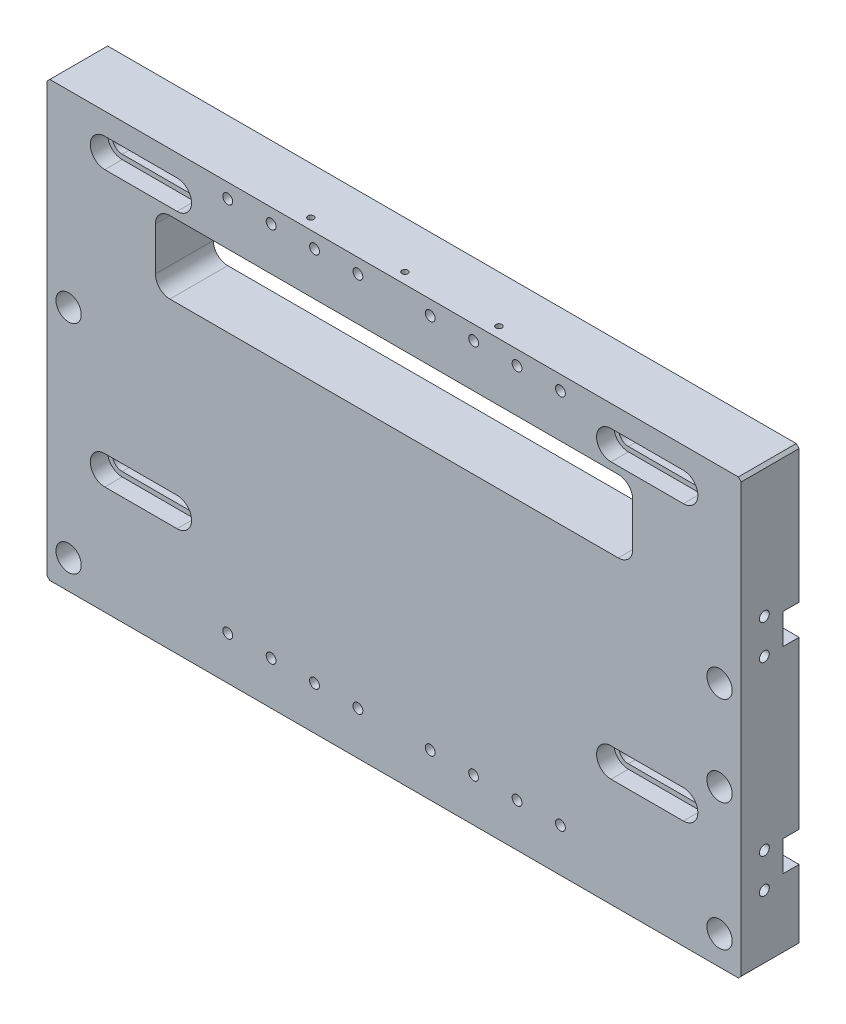
from build123d import *

# Parameters (mm, degrees)
SKETCH1_W                                            = 480
SKETCH1_H                                            = 300
BOSS_EXTRUDE1_DEPTH                                  = 20
CUT_EXTRUDE1_DEPTH                                   = 286.832118559
HOLE_SIZE_PER_SOCKET_HEAD_CAP_SCREW_TYPE_D           = 17.5
HOLE_SIZE_PER_SOCKET_HEAD_CAP_SCREW_TYPE_CBORE_D     = 26
HOLE_SIZE_PER_SOCKET_HEAD_CAP_SCREW_TYPE_CBORE_DEPTH = 17.5
CBORE_FOR_M12_HEX_SOCKET_HEAD_CAP_SCREW1_D           = 13.5
CBORE_FOR_M12_HEX_SOCKET_HEAD_CAP_SCREW1_CBORE_D     = 20
CBORE_FOR_M12_HEX_SOCKET_HEAD_CAP_SCREW1_CBORE_DEPTH = 12
SKETCH7_W                                            = 11
SKETCH7_H                                            = 21
CUT_EXTRUDE2_DEPTH                                   = 504.289181286
M5_TAPPED_HOLE1_D                                    = 4.2
M5_TAPPED_HOLE1_DEPTH                                = 12.4
M5_TAPPED_HOLE1_TIP                                  = 1.2618073
CUT_EXTRUDE5_START                                   = -100
CUT_EXTRUDE5_DEPTH                                   = 100
CUT_EXTRUDE6_DEPTH                                   = 12
CHAMFER1_SIZE                                        = 2
M8_TAPPED_HOLE1_D                                    = 6.8
M8_TAPPED_HOLE1_DEPTH                                = 19.75
M8_TAPPED_HOLE1_TIP                                  = 2.042926105
SKETCH29_R                                           = 11
CUT_EXTRUDE7_DEPTH                                   = 130
SKETCH30_R                                           = 14.25
CUT_EXTRUDE8_DEPTH                                   = 30
M6_TAPPED_HOLE2_D                                    = 5
M6_TAPPED_HOLE2_DEPTH                                = 15
M6_TAPPED_HOLE2_TIP                                  = 1.502151548
M8_TAPPED_HOLE2_AT_2_COUNT                           = 2
M8_TAPPED_HOLE2_AT_2_PITCH                           = 24
M8_TAPPED_HOLE2_AT_3_COUNT                           = 2
M8_TAPPED_HOLE2_AT_3_PITCH                           = 116
M8_TAPPED_HOLE2_AT_4_COUNT                           = 2
M8_TAPPED_HOLE2_AT_4_PITCH                           = 140


with BuildPart() as part:
    # Sketch1 → Boss-Extrude1 (new, symmetric)
    with BuildSketch(Plane.XY):
        Rectangle(SKETCH1_W, SKETCH1_H)
    extrude(amount=BOSS_EXTRUDE1_DEPTH, both=True)

    # Sketch2 → Cut-Extrude1 (cut, through all)
    with BuildSketch(Plane.XY.offset(20)):
        with BuildLine():
            Line((-155, 110), (155, 110))
            ThreePointArc((155, 110), (162.071067812, 107.071067812), (165, 100))
            Line((165, 100), (165, 70))
            ThreePointArc((165, 70), (162.071067812, 62.928932188), (155, 60))
            Line((155, 60), (-155, 60))
            ThreePointArc((-155, 60), (-162.071067812, 62.928932188), (-165, 70))
            Line((-165, 70), (-165, 100))
            ThreePointArc((-165, 100), (-162.071067812, 107.071067812), (-155, 110))
        make_face()
    extrude(amount=-CUT_EXTRUDE1_DEPTH, mode=Mode.SUBTRACT)

    # Hole size per socket head cap screw type2 (through all)
    with Locations(Plane(origin=(0, 0, -20), x_dir=(-1, 0, 0), z_dir=(0, 0, -1))):
        with Locations((-225, 20), (225, 20), (225, -130), (-225, -130), (-225, -42)):
            CounterBoreHole(HOLE_SIZE_PER_SOCKET_HEAD_CAP_SCREW_TYPE_D / 2, HOLE_SIZE_PER_SOCKET_HEAD_CAP_SCREW_TYPE_CBORE_D / 2, HOLE_SIZE_PER_SOCKET_HEAD_CAP_SCREW_TYPE_CBORE_DEPTH)

    # CBORE for M12 Hex Socket Head Cap Screw1 (through all)
    with Locations(Plane.XY.offset(20)):
        with Locations((-200, 125), (200, 125), (-200, -65), (200, -65)):
            CounterBoreHole(CBORE_FOR_M12_HEX_SOCKET_HEAD_CAP_SCREW1_D / 2, CBORE_FOR_M12_HEX_SOCKET_HEAD_CAP_SCREW1_CBORE_D / 2, CBORE_FOR_M12_HEX_SOCKET_HEAD_CAP_SCREW1_CBORE_DEPTH)

    # Sketch7 → Cut-Extrude2 (cut, through all)
    with BuildSketch(Plane.ZY.offset(240)):
        with Locations((-14.5, -90.5)):
            Rectangle(SKETCH7_W, SKETCH7_H)
        with Locations((-14.5, 45.5)):
            Rectangle(SKETCH7_W, SKETCH7_H)
    extrude(amount=-CUT_EXTRUDE2_DEPTH, mode=Mode.SUBTRACT)

    # M5 Tapped Hole1
    with Locations(Plane(origin=(0, 150, 0), x_dir=(-1, 0, 0), z_dir=(0, 1, 0))):
        with Locations((0, 12.5), (-65, 12.5), (65, 12.5)):
            Hole(M5_TAPPED_HOLE1_D / 2, depth=M5_TAPPED_HOLE1_DEPTH)
            with Locations((0, 0, -(M5_TAPPED_HOLE1_DEPTH + M5_TAPPED_HOLE1_TIP / 2))):  # 118° drill point
                Cone(0, M5_TAPPED_HOLE1_D / 2, M5_TAPPED_HOLE1_TIP, mode=Mode.SUBTRACT)

    # Sketch14 → Cut-Extrude5 (cut)
    with BuildSketch(Plane.XY.offset(8).offset(CUT_EXTRUDE5_START)):
        with BuildLine():
            Line((-200, 131.75), (-150, 131.75))
            ThreePointArc((-150, 131.75), (-143.25, 125), (-150, 118.25))
            Line((-150, 118.25), (-200, 118.25))
            ThreePointArc((-200, 118.25), (-206.75, 125), (-200, 131.75))
        make_face()
        with BuildLine():
            Line((-200, -58.25), (-150, -58.25))
            ThreePointArc((-150, -58.25), (-143.25, -65), (-150, -71.75))
            Line((-150, -71.75), (-200, -71.75))
            ThreePointArc((-200, -71.75), (-206.75, -65), (-200, -58.25))
        make_face()
        with BuildLine():
            Line((200, -71.75), (150, -71.75))
            ThreePointArc((150, -71.75), (143.25, -65), (150, -58.25))
            Line((150, -58.25), (200, -58.25))
            ThreePointArc((200, -58.25), (206.75, -65), (200, -71.75))
        make_face()
        with BuildLine():
            Line((200, 118.25), (150, 118.25))
            ThreePointArc((150, 118.25), (143.25, 125), (150, 131.75))
            Line((150, 131.75), (200, 131.75))
            ThreePointArc((200, 131.75), (206.75, 125), (200, 118.25))
        make_face()
    extrude(amount=CUT_EXTRUDE5_DEPTH, mode=Mode.SUBTRACT)

    # Sketch15 → Cut-Extrude6 (cut)
    with BuildSketch(Plane.XY.offset(20)):
        with BuildLine():
            Line((-200, 135), (-150, 135))
            ThreePointArc((-150, 135), (-140, 125), (-150, 115))
            Line((-150, 115), (-200, 115))
            ThreePointArc((-200, 115), (-210, 125), (-200, 135))
        make_face()
        with BuildLine():
            Line((-200, -55), (-150, -55))
            ThreePointArc((-150, -55), (-140, -65), (-150, -75))
            Line((-150, -75), (-200, -75))
            ThreePointArc((-200, -75), (-210, -65), (-200, -55))
        make_face()
        with BuildLine():
            Line((200, -75), (150, -75))
            ThreePointArc((150, -75), (140, -65), (150, -55))
            Line((150, -55), (200, -55))
            ThreePointArc((200, -55), (210, -65), (200, -75))
        make_face()
        with BuildLine():
            Line((200, 115), (150, 115))
            ThreePointArc((150, 115), (140, 125), (150, 135))
            Line((150, 135), (200, 135))
            ThreePointArc((200, 135), (210, 125), (200, 115))
        make_face()
    extrude(amount=-CUT_EXTRUDE6_DEPTH, mode=Mode.SUBTRACT)

    # Chamfer1
    chamfer1_edges = [part.edges().sort_by_distance(p)[0] for p in [
        (240, -150, 0),
        (-240, -150, 0),
        (-240, 150, 0),
        (240, 150, 0),
    ]]
    chamfer(chamfer1_edges, length=CHAMFER1_SIZE)

    # M8 Tapped Hole1
    with Locations(Plane.XY.offset(20)):
        with Locations((55, 140), (-55, -120), (55, -120), (-55, 140), (-25, 140), (25, 140), (-85, 140), (85, 140), (-25, -120), (-85, -120), (85, -120), (25, -120), (-115, -120), (115, -120), (-115, 140), (115, 140)):
            Hole(M8_TAPPED_HOLE1_D / 2, depth=M8_TAPPED_HOLE1_DEPTH)
            with Locations((0, 0, -(M8_TAPPED_HOLE1_DEPTH + M8_TAPPED_HOLE1_TIP / 2))):  # 118° drill point
                Cone(0, M8_TAPPED_HOLE1_D / 2, M8_TAPPED_HOLE1_TIP, mode=Mode.SUBTRACT)

    # Sketch29 → Cut-Extrude7 (cut)
    with BuildSketch(Plane.ZY.offset(240)):
        with Locations(Location((0, -20, 0), (0, 0, 270))):
            Circle(SKETCH29_R)
    extrude(amount=-CUT_EXTRUDE7_DEPTH, mode=Mode.SUBTRACT)

    # Sketch30 → Cut-Extrude8 (cut)
    with BuildSketch(Plane.ZY.offset(240)):
        with Locations(Location((0, -20, 0), (0, 0, 270))):
            Circle(SKETCH30_R)
    extrude(amount=-CUT_EXTRUDE8_DEPTH, mode=Mode.SUBTRACT)

    # M6 Tapped Hole2
    with Locations(Plane.ZY.offset(240)):
        with Locations((-10.5, -1.813466521), (10.5, -1.813466521), (10.5, -38.186533479), (-10.5, -38.186533479)):
            Hole(M6_TAPPED_HOLE2_D / 2, depth=M6_TAPPED_HOLE2_DEPTH)
            with Locations((0, 0, -(M6_TAPPED_HOLE2_DEPTH + M6_TAPPED_HOLE2_TIP / 2))):  # 118° drill point
                Cone(0, M6_TAPPED_HOLE2_D / 2, M6_TAPPED_HOLE2_TIP, mode=Mode.SUBTRACT)

    # Sketch34 → M8 Tapped Hole2 (revolve, cut)
    with BuildSketch(Plane(origin=(240, -80.5, 4), x_dir=(0, 0, -1), z_dir=(0, 1, 0))):
        Polygon((0, 0), (0, 24.292926105), (3.4, 22.25), (3.4, 0), align=None)
    m8_tapped_hole2 = revolve(axis=Axis((246.35, -80.5, 4), (-1, 0, 0)), mode=Mode.SUBTRACT)

    # M8 Tapped Hole2 at 2: M8 Tapped Hole2 ×2
    with Locations(*[(0, -i * M8_TAPPED_HOLE2_AT_2_PITCH, 0) for i in range(1, M8_TAPPED_HOLE2_AT_2_COUNT)]):
        add(m8_tapped_hole2, mode=Mode.SUBTRACT)

    # M8 Tapped Hole2 at 3: M8 Tapped Hole2 ×2
    with Locations(*[(0, i * M8_TAPPED_HOLE2_AT_3_PITCH, 0) for i in range(1, M8_TAPPED_HOLE2_AT_3_COUNT)]):
        add(m8_tapped_hole2, mode=Mode.SUBTRACT)

    # M8 Tapped Hole2 at 4: M8 Tapped Hole2 ×2
    with Locations(*[(0, i * M8_TAPPED_HOLE2_AT_4_PITCH, 0) for i in range(1, M8_TAPPED_HOLE2_AT_4_COUNT)]):
        add(m8_tapped_hole2, mode=Mode.SUBTRACT)

    # Mirror1: M8 Tapped Hole2 across plane
    add(m8_tapped_hole2.mirror(Plane(origin=(0, 0, 0), x_dir=(0, 0, 1), z_dir=(1, 0, 0))), mode=Mode.SUBTRACT)

    # Mirror1 copy 1 sketch → Mirror1 copy 1 (revolve, cut)
    with BuildSketch(Plane(origin=(-240, -104.5, 4), x_dir=(0, 0, -1), z_dir=(0, 1, 0))):
        Polygon((0, 0), (0, -24.292926105), (3.4, -22.25), (3.4, 0), align=None)
    revolve(axis=Axis((-246.35, -104.5, 4), (-1, 0, 0)), mode=Mode.SUBTRACT)

    # Mirror1 copy 2 sketch → Mirror1 copy 2 (revolve, cut)
    with BuildSketch(Plane(origin=(-240, 35.5, 4), x_dir=(0, 0, -1), z_dir=(0, 1, 0))):
        Polygon((0, 0), (0, -24.292926105), (3.4, -22.25), (3.4, 0), align=None)
    revolve(axis=Axis((-246.35, 35.5, 4), (-1, 0, 0)), mode=Mode.SUBTRACT)

    # Mirror1 copy 3 sketch → Mirror1 copy 3 (revolve, cut)
    with BuildSketch(Plane(origin=(-240, 59.5, 4), x_dir=(0, 0, -1), z_dir=(0, 1, 0))):
        Polygon((0, 0), (0, -24.292926105), (3.4, -22.25), (3.4, 0), align=None)
    revolve(axis=Axis((-246.35, 59.5, 4), (-1, 0, 0)), mode=Mode.SUBTRACT)


solid = part.part
